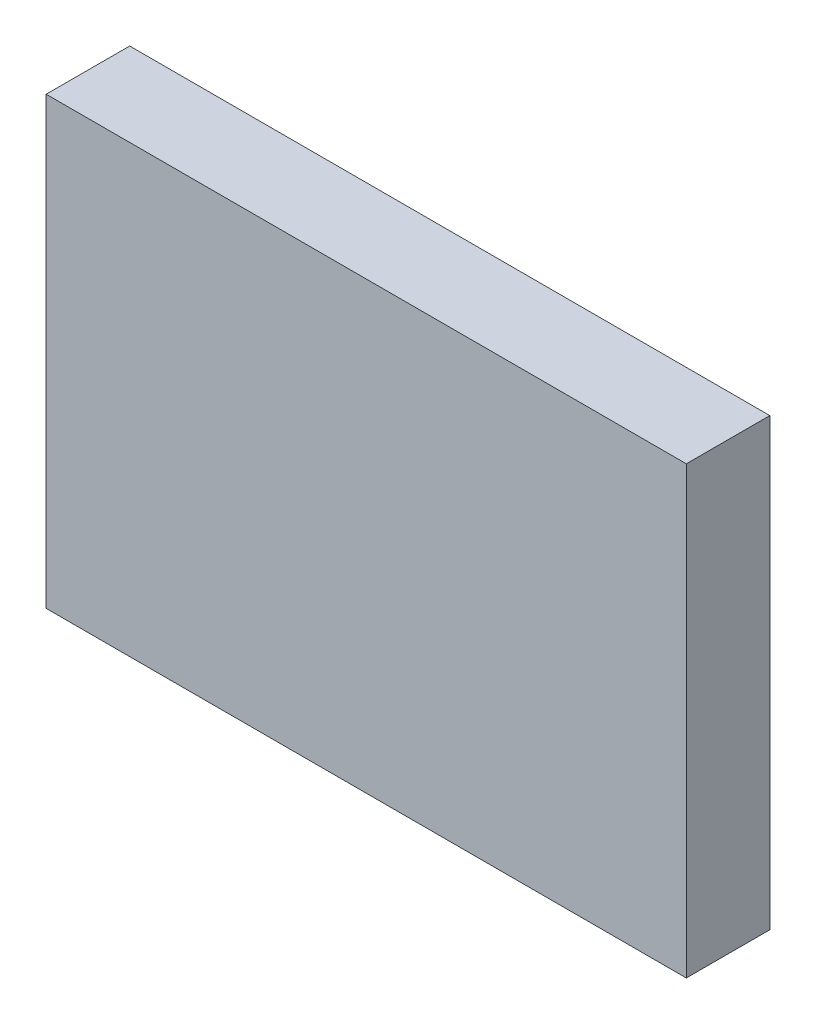
from build123d import *

# Parameters (mm, degrees)
SKETCH1_W           = 230
SKETCH1_H           = 160
BOSS_EXTRUDE1_DEPTH = 30


with BuildPart() as part:
    # Sketch1 → Boss-Extrude1 (new body)
    with BuildSketch(Plane.XY):
        with Locations((115, 80)):
            Rectangle(SKETCH1_W, SKETCH1_H)
    extrude(amount=BOSS_EXTRUDE1_DEPTH)


solid = part.part
